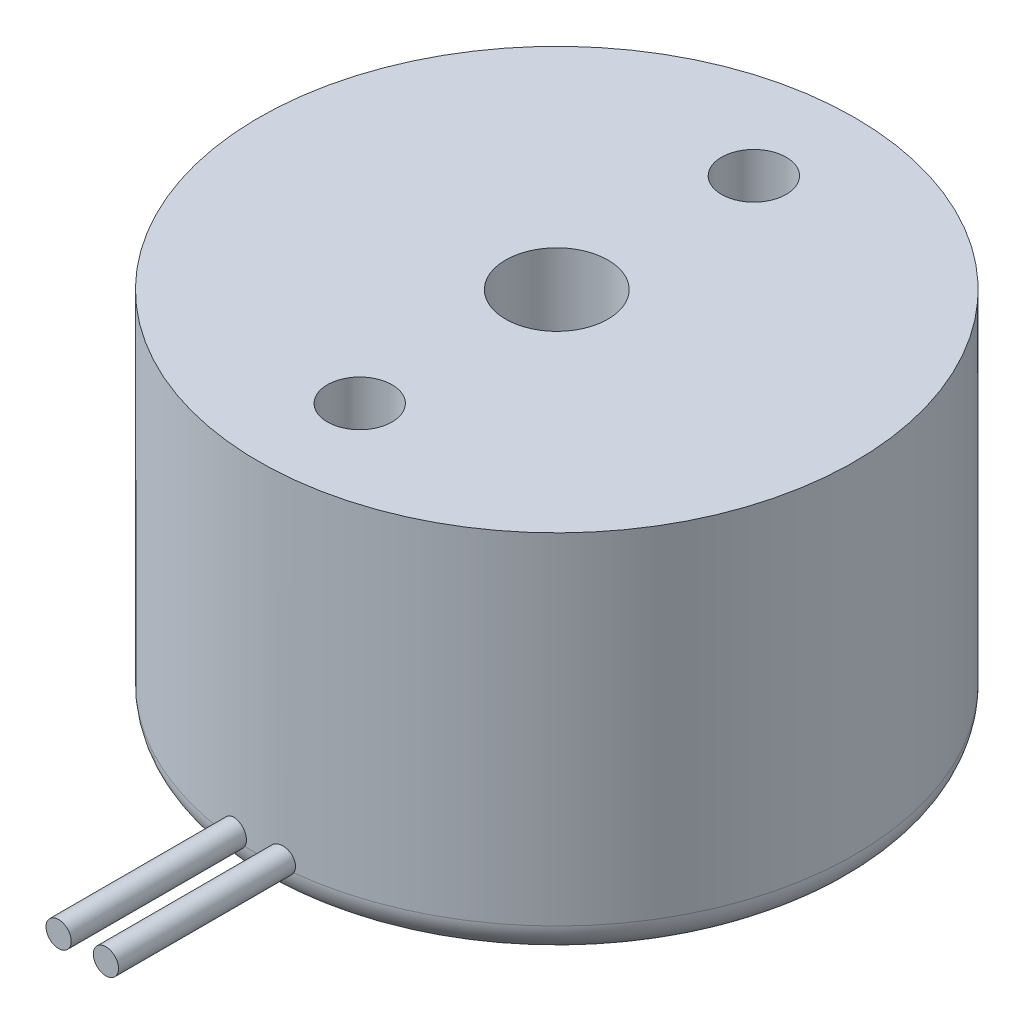
from build123d import *

# Parameters (mm, degrees)
M2_5_TAPPED_HOLE1_D     = 2.05
M2_5_TAPPED_HOLE1_DEPTH = 4.35
M2_5_TAPPED_HOLE1_TIP   = 0.615882135
SKETCH5_R               = 0.4
BOSS_EXTRUDE1_DEPTH     = 15
SKETCH6_R               = 4.15
CUT_EXTRUDE2_DEPTH      = 15


with BuildPart() as part:
    # Sketch1 → Revolve1 (revolve)
    with BuildSketch(Plane.XY, mode=Mode.PRIVATE) as revolve1_sk:
        with BuildLine():
            Line((1.625, 11.8), (9.45, 11.8))
            Line((9.45, 11.8), (9.45, 1))
            ThreePointArc((9.45, 1), (9.157106781, 0.292893219), (8.45, 0))
            Line((8.45, 0), (4.15, 0))
            Line((4.15, 0), (4.15, 6.3))
            Line((4.15, 6.3), (1.625, 6.3))
            Line((1.625, 6.3), (1.625, 11.8))
        make_face()
    revolve(revolve1_sk.sketch.rotate(Axis((0, 0, 0), (0, 1, 0)), 90), axis=Axis((0, 0, 0), (0, 1, 0)))

    # M2.5 Tapped Hole1
    with Locations(Plane(origin=(0, 11.8, 0), x_dir=(-1, 0, 0), z_dir=(0, 1, 0))):
        with Locations((0, -6.25), (0, 6.25)):
            Hole(M2_5_TAPPED_HOLE1_D / 2, depth=M2_5_TAPPED_HOLE1_DEPTH)
            with Locations((0, 0, -(M2_5_TAPPED_HOLE1_DEPTH + M2_5_TAPPED_HOLE1_TIP / 2))):  # 118° drill point
                Cone(0, M2_5_TAPPED_HOLE1_D / 2, M2_5_TAPPED_HOLE1_TIP, mode=Mode.SUBTRACT)

    # Sketch5 → Boss-Extrude1 (add)
    with BuildSketch(Plane.XY):
        with Locations(Location((-0.8, 1.2, 0), (0, 0, 180))):
            Circle(SKETCH5_R)
        with Locations(Location((0.7, 1.2, 0), (0, 0, 180))):
            Circle(SKETCH5_R)
    extrude(amount=BOSS_EXTRUDE1_DEPTH)

    # Sketch6 → Cut-Extrude2 (cut)
    with BuildSketch(Plane.XZ.offset(-6.3)):
        with Locations(Location((0, 0, 0), (0, 0, 270))):
            Circle(SKETCH6_R)
    extrude(amount=CUT_EXTRUDE2_DEPTH, mode=Mode.SUBTRACT)


solid = part.part
